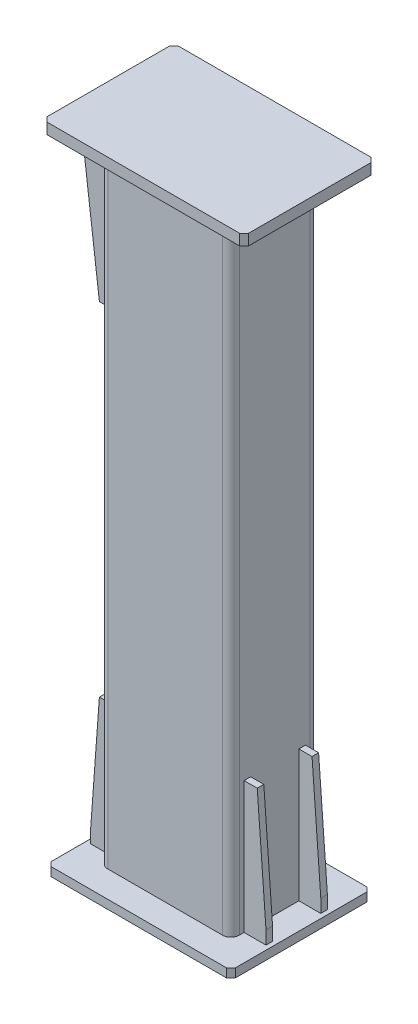
SolidWorks part; units mm, degrees
ref_plane "Front Plane" through (0, 0, 0) normal (0, 0, 1) x (1, 0, 0)
ref_plane "Top Plane" through (0, 0, 0) normal (0, 1, 0) x (1, 0, 0)
ref_plane "Right Plane" through (0, 0, 0) normal (1, 0, 0) x (0, 0, -1)
sketch "Sketch1" plane through (0, 0, 0) normal (0, 1, 0) x (1, 0, 0)
  line L0 (0, 310) -> (10, 320)
  line L1 (10, 0) -> (410, 0)
  line L2 (0, 10) -> (0, 310)
  line L3 (10, 320) -> (410, 320)
  line L4 (420, 10) -> (420, 310)
  line L5 (10, 0) -> (0, 10)
  line L6 (410, 0) -> (420, 10)
  line L7 (420, 310) -> (410, 320)
  point P0 (0, 0)
  point P1 (420, 320)
  point P2 (0, 320)
  point P3 (420, 0)
  dimension "D1" = 420
  dimension "D2" = 320
extrude "Boss-Extrude1" add sketch "Sketch1" along normal blind 20
sketch "Sketch2" plane through (0, 20, 0) normal (0, 1, 0) x (1, 0, 0)
  line L0 (410, 320) -> (10, 320) construction
  line L1 (79.0709, 260) -> (340.9291, 260)
  line L2 (60, 240.9291) -> (60, 79.0709)
  line L3 (79.0709, 60) -> (340.9291, 60)
  line L4 (360, 240.9291) -> (360, 79.0709)
  line L5 (0, 310) -> (0, 10) construction
  line L6 (60, 160) -> (326.366, 160) construction
  line L7 (79.0709, 252) -> (340.9291, 252)
  line L8 (352, 240.9291) -> (352, 79.0709)
  line L9 (79.0709, 68) -> (340.9291, 68)
  line L10 (68, 240.9291) -> (68, 79.0709)
  arc A0 (340.9291, 260) -> (360, 240.9291) centre (340.9291, 240.9291) cw
  arc A1 (360, 79.0709) -> (340.9291, 60) centre (340.9291, 79.0709) cw
  arc A2 (79.0709, 60) -> (60, 79.0709) centre (79.0709, 79.0709) cw
  arc A3 (60, 240.9291) -> (79.0709, 260) centre (79.0709, 240.9291) cw
  arc A4 (340.9291, 252) -> (352, 240.9291) centre (340.9291, 240.9291) cw
  arc A5 (352, 79.0709) -> (340.9291, 68) centre (340.9291, 79.0709) cw
  arc A6 (79.0709, 68) -> (68, 79.0709) centre (79.0709, 79.0709) cw
  arc A7 (68, 240.9291) -> (79.0709, 252) centre (79.0709, 240.9291) cw
  dimension "D5" = 19.0709
  dimension "D1" = 300
  dimension "D2" = 200
  dimension "D3" = 60
  dimension "D4" = 60
  dimension "D6" = 8
extrude "Boss-Extrude2" add sketch "Sketch2" along normal blind 1431
sketch "Sketch3" plane through (0, 1451, 0) normal (0, 1, 0) x (1, 0, 0)
  line L0 (340.9291, 260) -> (79.0709, 260) construction
  line L1 (-10, 310) -> (430, 310)
  line L2 (-20, 300) -> (-20, 20)
  line L3 (-10, 10) -> (430, 10)
  line L4 (440, 300) -> (440, 20)
  line L6 (440, 20) -> (430, 10)
  line L7 (-20, 20) -> (-10, 10)
  line L8 (-10, 310) -> (-20, 300)
  line L9 (430, 310) -> (440, 300)
  line L10 (60, 240.9291) -> (60, 79.0709) construction
  point P0 (-20, 310)
  point P1 (440, 10)
  point P2 (-20, 10)
  point P3 (440, 310)
  dimension "D1" = 460
  dimension "D2" = 300
  dimension "D3" = 50
  dimension "D4" = 80
extrude "Boss-Extrude3" add sketch "Sketch3" along normal blind 25
ref_plane "Plane1" through (0, 0, -160) normal (0, 0, 1) x (1, 0, 0)
sketch "Sketch4" plane through (0, 0, -260) normal (0, 0, -1) x (-1, 0, 0)
  line L1 (-30, 320) -> (-10, 50)
  line L2 (-30, 320) -> (-390, 320)
  line L4 (-10, 50) -> (-10, 20)
  line L5 (-410, 50) -> (-410, 20)
  line L6 (-420, 20) -> (-410, 20) construction
  line L7 (-410, 20) -> (-10, 20)
  line L10 (-410, 50) -> (-390, 320)
  line L11 (-360, 1451) -> (-360, 20) construction
  line L12 (-420, 20) -> (-420, 0) construction
  point P3 (-420, 10)
  point P5 (-46.9319, 506.3413)
  point P6 (-360, 320)
  dimension "D6" = 360
  dimension "D1" = 300
  dimension "D2" = 30
  dimension "D3" = 30
  dimension "D4" = 10
  dimension "D5" = 400
extrude "Boss-Extrude4" add sketch "Sketch4" against normal blind 15 from offset 30 offset against normal yes
mirror "Mirror1" about plane through (0, 0, -160) normal (0, 0, 1) of "Boss-Extrude4"
sketch "Sketch5" plane through (0, 0, -60) normal (0, 0, 1) x (1, 0, 0)
  line L0 (60, 1441) -> (50, 1451)
  line L5 (-10, 1451) -> (430, 1451) construction
  line L9 (60, 1101) -> (60, 1441)
  line L11 (60, 1451) -> (60, 20) construction
  line L12 (50, 1451) -> (-10, 1451)
  line L13 (-10, 1451) -> (-10, 1421)
  line L14 (-10, 1421) -> (30, 1101)
  line L15 (30, 1101) -> (60, 1101)
  line L16 (-20, 1476) -> (-20, 1451) construction
  point P15 (60, 1451)
  point P19 (-20, 1463.5)
  dimension "D6" = 30
  dimension "D7" = 30
  dimension "D8" = 10
  dimension "D9" = 350
ref_plane "Plane2" through (210, 0, 0) normal (1, 0, 0) x (0, 0, -1)
extrude "Boss-Extrude7" add sketch "Sketch5" against normal blind 15 from offset 30 offset against normal yes
mirror "Mirror5" about plane through (0, 0, -160) normal (0, 0, 1) of "Boss-Extrude7"
